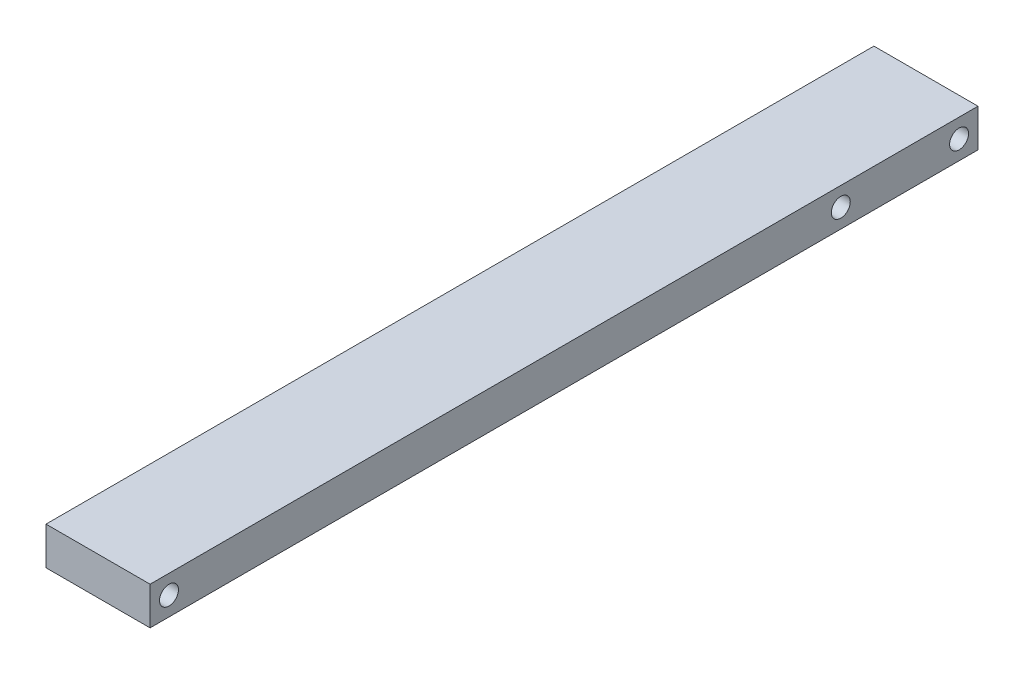
SolidWorks part; units mm, degrees
ref_plane "Front Plane" through (0, 0, 0) normal (0, 0, 1) x (1, 0, 0)
ref_plane "Top Plane" through (0, 0, 0) normal (0, 1, 0) x (1, 0, 0)
ref_plane "Right Plane" through (0, 0, 0) normal (1, 0, 0) x (0, 0, -1)
sketch "Sketch1" plane through (0, 0, 0) normal (0, 0, 1) x (1, 0, 0)
  line L1 (0, 0) -> (22, 0)
  line L2 (0, 0) -> (0, 8)
  line L3 (0, 8) -> (22, 8)
  line L4 (22, 0) -> (22, 8)
  dimension "D1" = 22
  dimension "D2" = 8
extrude "Boss-Extrude1" add sketch "Sketch1" along normal blind 175
sketch "Sketch2" plane through (22, 0, 0) normal (1, 0, 0) x (0, 0, -1)
  line L0 (0, 0) -> (0, 8) construction
  line L1 (-175, 0) -> (-175, 8) construction
  circle A0 centre (-4, 4) radius 2
  circle A1 centre (-171, 4) radius 2
  circle A2 centre (-29, 4) radius 2
  dimension "D1" = 4
  dimension "D3" = 4
  dimension "D5" = 4
  dimension "D2" = 4
  dimension "D4" = 4
  dimension "D6" = 25
extrude "Cut-Extrude1" cut sketch "Sketch2" against normal through all
